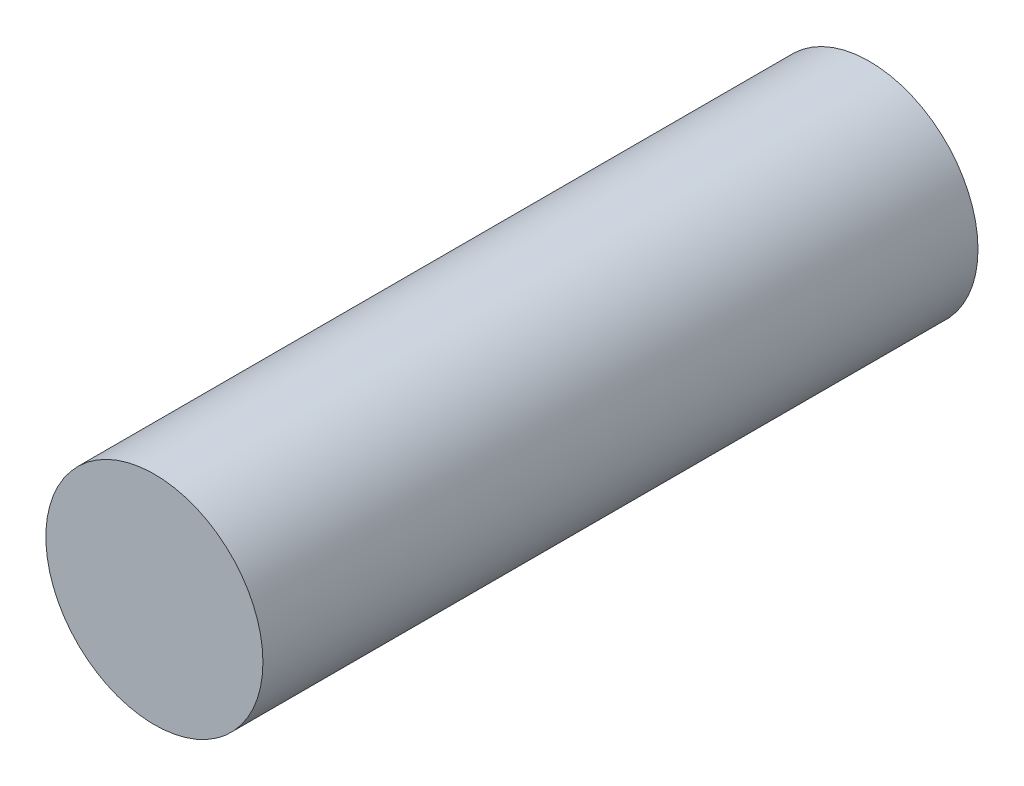
from build123d import *

# Parameters (mm, degrees)
SKETCH1_R           = 40
BOSS_EXTRUDE1_DEPTH = 263.5


with BuildPart() as part:
    # Sketch1 → Boss-Extrude1 (new body)
    with BuildSketch(Plane.XY):
        Circle(SKETCH1_R)
    extrude(amount=BOSS_EXTRUDE1_DEPTH)


solid = part.part
